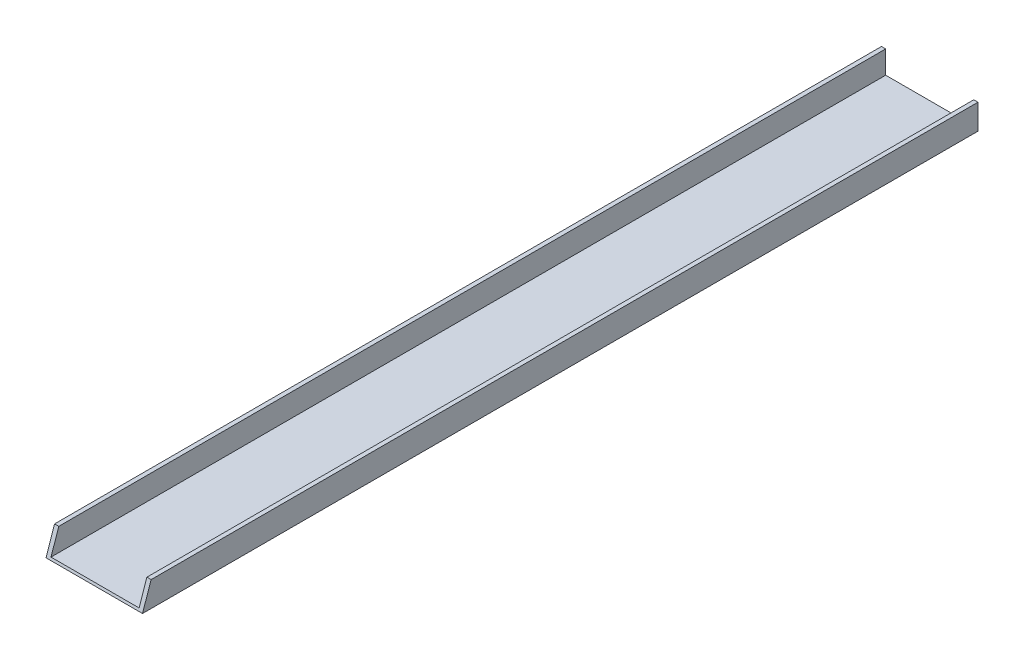
SolidWorks part; units mm, degrees
material "AISI 1045 钢，冷拔"
ref_plane "Front Plane" through (0, 0, 0) normal (0, 0, 1) x (1, 0, 0)
ref_plane "Top Plane" through (0, 0, 0) normal (0, 1, 0) x (1, 0, 0)
ref_plane "Right Plane" through (0, 0, 0) normal (1, 0, 0) x (0, 0, -1)
sketch "Sketch1" plane through (0, 0, 0) normal (0, 0, 1) x (1, 0, 0)
  line L0 (127, 0) -> (-127, 0)
  line L1 (55, 0) -> (-55, 0) construction
  line L2 (-127, 0) -> (-127, 66.04)
  line L3 (-127, 66.04) -> (-115.9256, 66.04)
  line L4 (-115.9256, 66.04) -> (-115.9256, 6.096)
  line L5 (-115.9256, 6.096) -> (115.9256, 6.096)
  line L6 (115.9256, 6.096) -> (115.9256, 66.04)
  line L7 (115.9256, 66.04) -> (127, 66.04)
  line L8 (127, 66.04) -> (127, 0)
  line L9 (0, -55) -> (0, 55) construction
  dimension "D1" = 254
  dimension "D2" = 127
  dimension "D3" = 66.04
  dimension "D4" = 11.0744
  dimension "D5" = 6.096
extrude "Boss-Extrude1" add sketch "Sketch1" along normal mid plane 2198.675
sketch "Sketch2" plane through (0, 0, 0) normal (1, 0, 0) x (0, 0, -1)
  line L0 (-1099.3375, 0) -> (-1076.7527, 66.04)
  line L1 (139.7, 0) -> (-139.7, 0) construction
  line L2 (-1099.3375, 0) -> (-1099.3375, 66.04) construction
  line L3 (-1099.3375, 66.04) -> (1099.3375, 66.04) construction
  line L4 (-1076.7527, 66.04) -> (-1099.3375, 66.04)
  line L5 (-1099.3375, 66.04) -> (-1099.3375, 0)
  dimension "D1" = 18.88
extrude "Cut-Extrude1" cut sketch "Sketch2" against normal mid plane 300
